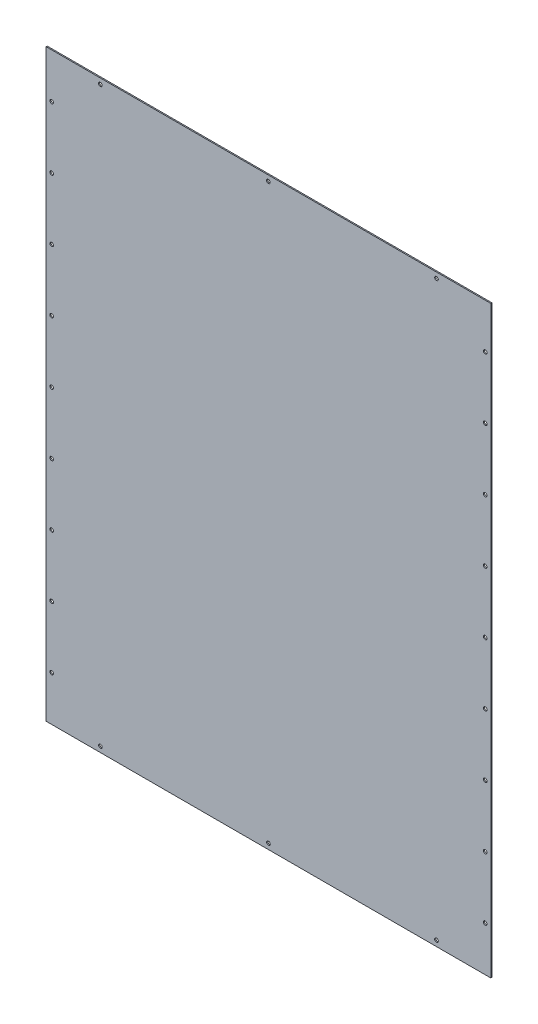
from build123d import *

# Parameters (mm, degrees)
SKETCH_1_W      = 794
SKETCH_1_H      = 1043
SKETCH_1_R      = 3.25
EXTRUDE_1_DEPTH = 2


with BuildPart() as part:
    # 草图1 → 凸台-拉伸1 (new body)
    with BuildSketch(Plane.XY):
        Rectangle(SKETCH_1_W, SKETCH_1_H)
        with Locations((-387, 0)):
            Circle(SKETCH_1_R, mode=Mode.SUBTRACT)
        with Locations((-387, -110.375)):
            Circle(SKETCH_1_R, mode=Mode.SUBTRACT)
        with Locations((-387, -220.75)):
            Circle(SKETCH_1_R, mode=Mode.SUBTRACT)
        with Locations((-387, -331.125)):
            Circle(SKETCH_1_R, mode=Mode.SUBTRACT)
        with Locations((-387, -441.5)):
            Circle(SKETCH_1_R, mode=Mode.SUBTRACT)
        with Locations((0, -511.5)):
            Circle(SKETCH_1_R, mode=Mode.SUBTRACT)
        with Locations(Location((0, 511.5, 0), (0, 0, 180))):
            Circle(SKETCH_1_R, mode=Mode.SUBTRACT)
        with Locations(Location((-387, 441.5, 0), (0, 0, 180))):
            Circle(SKETCH_1_R, mode=Mode.SUBTRACT)
        with Locations(Location((-387, 331.125, 0), (0, 0, 180))):
            Circle(SKETCH_1_R, mode=Mode.SUBTRACT)
        with Locations(Location((-387, 220.75, 0), (0, 0, 180))):
            Circle(SKETCH_1_R, mode=Mode.SUBTRACT)
        with Locations(Location((-387, 110.375, 0), (0, 0, 180))):
            Circle(SKETCH_1_R, mode=Mode.SUBTRACT)
        with Locations((387, 110.375)):
            Circle(SKETCH_1_R, mode=Mode.SUBTRACT)
        with Locations((387, 220.75)):
            Circle(SKETCH_1_R, mode=Mode.SUBTRACT)
        with Locations((387, 331.125)):
            Circle(SKETCH_1_R, mode=Mode.SUBTRACT)
        with Locations((387, 441.5)):
            Circle(SKETCH_1_R, mode=Mode.SUBTRACT)
        with Locations(Location((387, -441.5, 0), (0, 0, 180))):
            Circle(SKETCH_1_R, mode=Mode.SUBTRACT)
        with Locations(Location((387, -331.125, 0), (0, 0, 180))):
            Circle(SKETCH_1_R, mode=Mode.SUBTRACT)
        with Locations(Location((387, -220.75, 0), (0, 0, 180))):
            Circle(SKETCH_1_R, mode=Mode.SUBTRACT)
        with Locations(Location((387, -110.375, 0), (0, 0, 180))):
            Circle(SKETCH_1_R, mode=Mode.SUBTRACT)
        with Locations(Location((387, 0, 0), (0, 0, 180))):
            Circle(SKETCH_1_R, mode=Mode.SUBTRACT)
        with Locations((-300, 511.5)):
            Circle(SKETCH_1_R, mode=Mode.SUBTRACT)
        with Locations((300, 511.5)):
            Circle(SKETCH_1_R, mode=Mode.SUBTRACT)
        with Locations(Location((300, -511.5, 0), (0, 0, 180))):
            Circle(SKETCH_1_R, mode=Mode.SUBTRACT)
        with Locations(Location((-300, -511.5, 0), (0, 0, 180))):
            Circle(SKETCH_1_R, mode=Mode.SUBTRACT)
    extrude(amount=EXTRUDE_1_DEPTH)


solid = part.part
